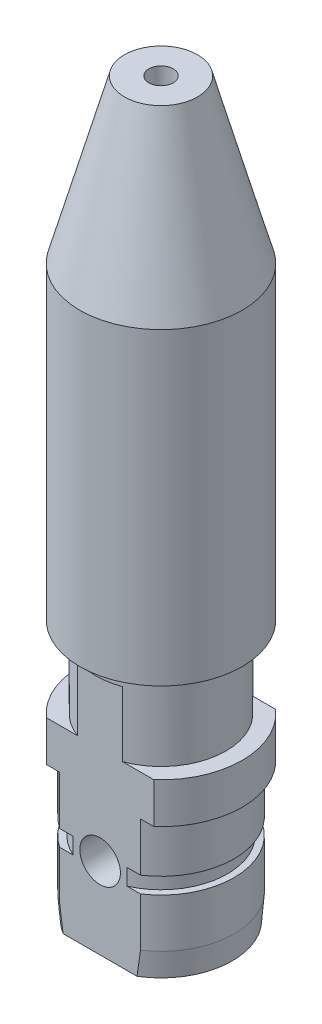
from build123d import *

# Parameters (mm, degrees)
SKETCH2_OUTSIDE_W   = 40.868
SKETCH2_OUTSIDE_H   = 40.868
SKETCH2_OUTSIDE_W_2 = 26.310212334
SKETCH2_OUTSIDE_H_2 = 15
CUT_EXTRUDE1_DEPTH  = 30
SKETCH3_R           = 2.5
CUT_EXTRUDE2_DEPTH  = 5
CUT_EXTRUDE3_START  = -5
SKETCH5_R           = 2.5
CUT_EXTRUDE3_DEPTH  = 5


with BuildPart() as part:
    # Sketch1 → Revolve1 (revolve)
    with BuildSketch(Plane.XY, mode=Mode.PRIVATE) as revolve1_sk:
        Polygon((-1.5, -45.854266644), (-1.5, 44.145733356), (-4.5, 44.145733356), (-10, 24.145733356), (-10, -13.854266644), (-8, -13.854266644), (-8, -23.854266644), (-10, -23.854266644), (-10, -28.854266644), (-9, -28.854266644), (-9, -34.854266644), (-8.2, -34.854266644), (-8.2, -36.854266644), (-9, -36.854266644), (-9, -42.854266644), (-8.77234172, -45.854266644), align=None)
    revolve(revolve1_sk.sketch.rotate(Axis((0, 0, 0), (0, 1, 0)), 270), axis=Axis((0, 0, 0), (0, 1, 0)))

    # Sketch2 outside → Cut-Extrude1 (cut)
    with BuildSketch(Plane(origin=(0, -45.854266644, 0), x_dir=(-1, 0, 0), z_dir=(0, -1, 0))):
        Rectangle(SKETCH2_OUTSIDE_W, SKETCH2_OUTSIDE_H)
        Rectangle(SKETCH2_OUTSIDE_W_2, SKETCH2_OUTSIDE_H_2, mode=Mode.SUBTRACT)
    extrude(amount=-CUT_EXTRUDE1_DEPTH, mode=Mode.SUBTRACT)

    # Sketch3 → Cut-Extrude2 (cut)
    with BuildSketch(Plane.XY.offset(7.5)):
        with Locations((0, -35.854266644)):
            Circle(SKETCH3_R)
    extrude(amount=-CUT_EXTRUDE2_DEPTH, mode=Mode.SUBTRACT)

    # Sketch5 → Cut-Extrude3 (cut)
    with BuildSketch(Plane(origin=(0, 0, -7.5), x_dir=(-1, 0, 0), z_dir=(0, 0, -1)).offset(CUT_EXTRUDE3_START)):
        with Locations(Location((0, -35.854266644, 0), (0, 0, 180))):
            Circle(SKETCH5_R)
    extrude(amount=CUT_EXTRUDE3_DEPTH, mode=Mode.SUBTRACT)


solid = part.part
